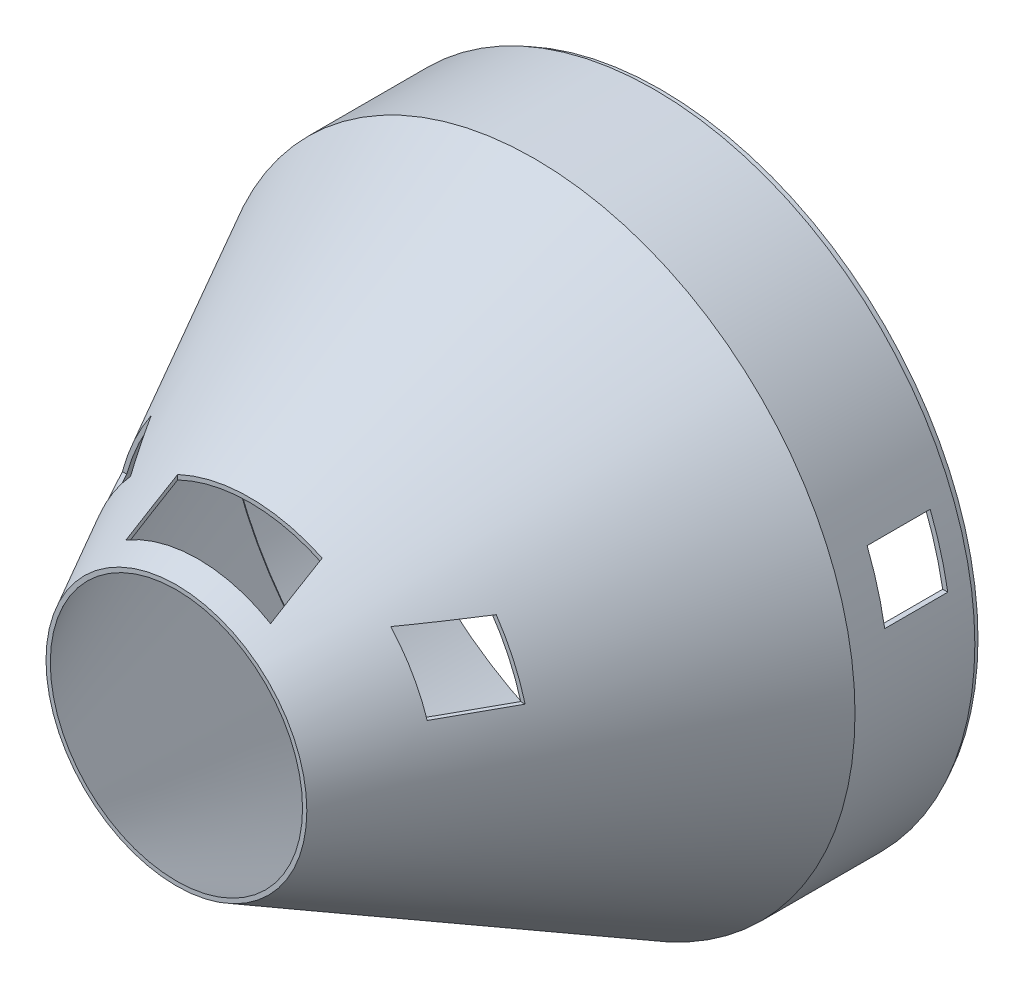
SolidWorks part; units mm, degrees
material "AISI 304"
ref_plane "Front Plane" through (0, 0, 0) normal (0, 0, 1) x (1, 0, 0)
ref_plane "Top Plane" through (0, 0, 0) normal (0, 1, 0) x (1, 0, 0)
ref_plane "Right Plane" through (0, 0, 0) normal (1, 0, 0) x (0, 0, -1)
sketch "Sketch2" plane through (0, 0, 0) normal (0, 0, 1) x (1, 0, 0)
  circle A0 centre (0, 0) radius 250
  circle A1 centre (0, 0) radius 254
  dimension "D1" = 500
  dimension "D2" = 508
extrude "Boss-Extrude1" add sketch "Sketch2" along normal blind 100
ref_plane "Plane1" through (0, 0, 384) normal (0, 0, 1) x (1, 0, 0)
sketch "Sketch5" plane through (0, 0, 0) normal (0, 1, 0) x (1, 0, 0)
  line L0 (0, 0) -> (0, -485.6691) construction
  line L1 (254, -100) -> (103.3957, -384)
  line L2 (-279.4, -384) -> (279.4, -384) construction
  line L3 (250.6043, -100) -> (100, -384)
  line L4 (-254, -100) -> (254, -100) construction
  line L5 (250.6043, -100) -> (254, -100)
  line L6 (100, -384) -> (103.3957, -384)
  dimension "D1" = 3
  dimension "D2" = 100
revolve "Revolve1" add sketch "Sketch5" angle 360 about L0
sketch "Sketch7" plane through (0, 0, 0) normal (1, 0, 0) x (0, 0, -1)
  line L1 (-72.8, 92.9) -> (-22.8, 92.9)
  line L2 (-72.8, 92.9) -> (-72.8, 42.9)
  line L3 (-72.8, 42.9) -> (-22.8, 42.9)
  line L4 (-22.8, 92.9) -> (-22.8, 42.9)
  line L5 (-317.2, 92.9) -> (-267.2, 92.9)
  line L6 (-317.2, 92.9) -> (-317.2, 42.9)
  line L7 (-317.2, 42.9) -> (-267.2, 42.9)
  line L8 (-267.2, 92.9) -> (-267.2, 42.9)
extrude "Cut-Extrude3" cut sketch "Sketch7" against normal mid plane 1000
sketch "Sketch8" plane through (0, 0, 0) normal (0, 0, -1) x (-1, 0, 0)
  circle A0 centre (0, 0) radius 254
  circle A1 centre (0, 0) radius 251.5
  dimension "D1" = 503
extrude "Cut-Extrude4" cut sketch "Sketch8" against normal blind 5
sketch "Sketch9" plane through (600, 66.2335, 45.3003) normal (0, 1, 0) x (1, 0, 0)
  line L1 (-657.2168, -280.5098) -> (-542.5932, -280.5098)
  line L2 (-657.2168, -280.5098) -> (-657.2168, -321.4468)
  line L3 (-657.2168, -321.4468) -> (-542.5932, -321.4468)
  line L4 (-542.5932, -280.5098) -> (-542.5932, -321.4468)
extrude "Cut-Extrude5" cut sketch "Sketch9" against normal blind 200 from offset 100
